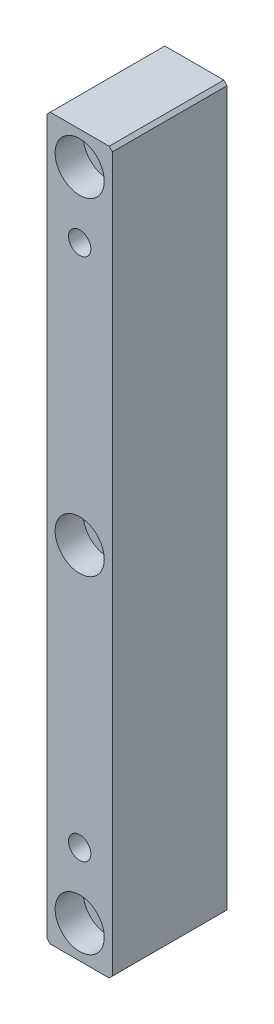
SolidWorks part; units mm, degrees
material "6061Al"
ref_plane "前视基准面" through (0, 0, 0) normal (0, 0, 1) x (1, 0, 0)
ref_plane "上视基准面" through (0, 0, 0) normal (0, 1, 0) x (1, 0, 0)
ref_plane "右视基准面" through (0, 0, 0) normal (1, 0, 0) x (0, 0, -1)
sketch "草图1" plane through (0, 0, 0) normal (0, 0, 1) x (1, 0, 0)
  line L1 (-10, -110) -> (10, -110)
  line L2 (-10, -110) -> (-10, 110)
  line L3 (-10, 110) -> (10, 110)
  line L4 (10, -110) -> (10, 110)
  line L5 (-10, -110) -> (10, 110) construction
  line L6 (-10, 110) -> (10, -110) construction
  point P0 (0, 0)
  dimension "D1" = 220
  dimension "D2" = 20
extrude "凸台-拉伸1" add sketch "草图1" along normal mid plane 35
hole_wizard "M8 六角凹头螺钉的柱形沉头孔1" positions "草图2" profile "草图3" counterbore size "M8" standard "ISO" end condition through all
sketch "草图2" plane through (0, 0, 17.5) normal (0, 0, 1) x (1, 0, 0)
  line L0 (0, 0) -> (73.8049, 0) construction
  point P0 (0, 100)
  point P2 (0, 0)
  point P5 (0, -100)
  dimension "D1" = 200
sketch "草图3" plane through (0, 100, 17.5) normal (1, 0, 0) x (0, -1, 0)
  line L0 (0, 0) -> (0, 35)
  line L1 (0, 35) -> (4.5, 35)
  line L3 (4.5, 35) -> (4.5, 8.6)
  line L4 (4.5, 8.6) -> (7.5, 8.6)
  line L5 (7.5, 8.6) -> (7.5, 0)
  line L7 (7.5, 0) -> (0, 0)
  line L11 (0, -6.35) -> (0, 107.95) construction
  dimension "通孔孔直径" = 9
  dimension "通孔孔深度" = 35
  dimension "柱形沉头孔直径" = 15
  dimension "柱形沉头孔深度" = 8.6
hole_wizard "M8 螺纹孔1" positions "草图4" profile "草图5" tap size "M8" standard "ISO"
sketch "草图4" plane through (0, 0, 17.5) normal (0, 0, 1) x (1, 0, 0)
  line L0 (0, 0) -> (56.7252, 0) construction
  point P0 (0, 80)
  point P2 (0, -80)
  dimension "D1" = 160
sketch "草图5" plane through (0, 80, 17.5) normal (1, 0, 0) x (0, -1, 0)
  line L0 (0, 0) -> (0, 21.7929)
  line L1 (0, 21.7929) -> (3.4, 19.75)
  line L2 (3.4, 19.75) -> (3.4, 0)
  line L5 (3.4, 0) -> (0, 0)
  line L10 (0, 21.7929) -> (-3.4, 19.75) construction
  line L11 (0, -6.35) -> (0, 107.95) construction
  dimension "螺纹孔钻头直径" = 6.8
  dimension "螺纹孔钻头深度" = 19.75
  dimension "导头角度" = 118
cosmetic thread "孔螺蚊线1" parameters "D1"=16, "D2"=8
cosmetic thread "孔螺蚊线2" parameters "D1"=16, "D2"=8
chamfer "倒角1" distance 1 angle 45 4 edges at (-10, -110, 0) (10, -110, 0) (10, 110, 0) (-10, 110, 0)
